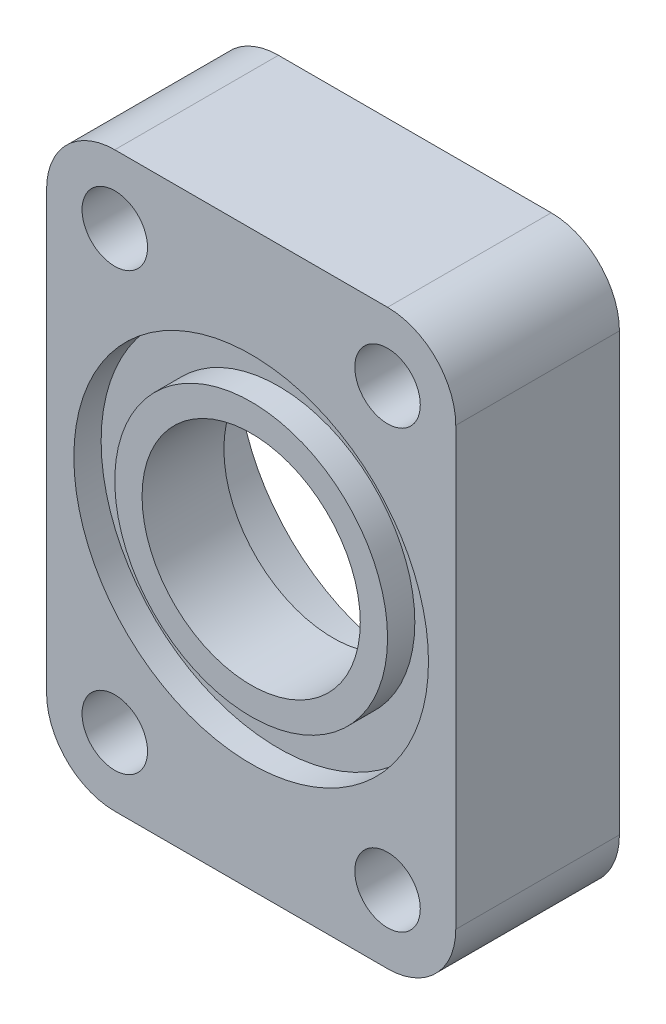
from build123d import *

# Parameters (mm, degrees)
SKETCH1_R           = 4
BOSS_EXTRUDE1_DEPTH = 6
SKETCH3_R           = 6.5
CUT_EXTRUDE2_DEPTH  = 3
CUT_EXTRUDE3_START  = -1
SKETCH4_R           = 6.5
SKETCH4_R_2         = 5
CUT_EXTRUDE3_DEPTH  = 1
SKETCH5_W           = 15
SKETCH5_H           = 3
BOSS_EXTRUDE2_DEPTH = 6
SKETCH6_R           = 1.2
CUT_EXTRUDE7_DEPTH  = 17
FILLET3_R           = 2.5
SKETCH7_R           = 2.2
CUT_EXTRUDE8_DEPTH  = 4


with BuildPart() as part:
    # Sketch1 → Boss-Extrude1 (new body)
    with BuildSketch(Plane.XY):
        Polygon((7.5, 0), (7.5, 7.5), (-7.5, 7.5), (-7.5, -7.5), (7.5, -7.5), align=None)
        Circle(SKETCH1_R, mode=Mode.SUBTRACT)
    extrude(amount=BOSS_EXTRUDE1_DEPTH)

    # Sketch3 → Cut-Extrude2 (cut)
    with BuildSketch(Plane(origin=(0, 0, 0), x_dir=(-1, 0, 0), z_dir=(0, 0, -1))):
        Circle(SKETCH3_R)
    extrude(amount=-CUT_EXTRUDE2_DEPTH, mode=Mode.SUBTRACT)

    # Sketch4 → Cut-Extrude3 (cut)
    with BuildSketch(Plane.XY.offset(6).offset(CUT_EXTRUDE3_START)):
        with Locations(Location((0, 0, 0), (0, 0, 180))):
            Circle(SKETCH4_R)
        Circle(SKETCH4_R_2, mode=Mode.SUBTRACT)
    extrude(amount=CUT_EXTRUDE3_DEPTH, mode=Mode.SUBTRACT)

    # Sketch5 → Boss-Extrude2 (add)
    with BuildSketch(Plane(origin=(0, 0, 0), x_dir=(-1, 0, 0), z_dir=(0, 0, -1))):
        with Locations((0, -9)):
            Rectangle(SKETCH5_W, SKETCH5_H)
        with Locations((0, 9)):
            Rectangle(SKETCH5_W, SKETCH5_H)
    extrude(amount=-BOSS_EXTRUDE2_DEPTH)

    # Sketch6 → Cut-Extrude7 (cut)
    with BuildSketch(Plane(origin=(0, 0, 0), x_dir=(-1, 0, 0), z_dir=(0, 0, -1))):
        with Locations((5, 8)):
            Circle(SKETCH6_R)
        with Locations((-5, 8)):
            Circle(SKETCH6_R)
        with Locations((-5, -8)):
            Circle(SKETCH6_R)
        with Locations((5, -8)):
            Circle(SKETCH6_R)
    extrude(amount=-CUT_EXTRUDE7_DEPTH, mode=Mode.SUBTRACT)

    # Fillet3
    fillet3_edges = [part.edges().sort_by_distance(p)[0] for p in [
        (-7.5, -10.5, 3),
        (7.5, -10.5, 3),
        (7.5, 10.5, 3),
        (-7.5, 10.5, 3),
    ]]
    fillet(fillet3_edges, radius=FILLET3_R)

    # Sketch7 → Cut-Extrude8 (cut)
    with BuildSketch(Plane(origin=(0, 0, 0), x_dir=(-1, 0, 0), z_dir=(0, 0, -1))):
        with Locations((-5, -8)):
            Circle(SKETCH7_R)
        with Locations((-5, 8)):
            Circle(SKETCH7_R)
        with Locations((5, 8)):
            Circle(SKETCH7_R)
        with Locations((5, -8)):
            Circle(SKETCH7_R)
    extrude(amount=-CUT_EXTRUDE8_DEPTH, mode=Mode.SUBTRACT)


solid = part.part
